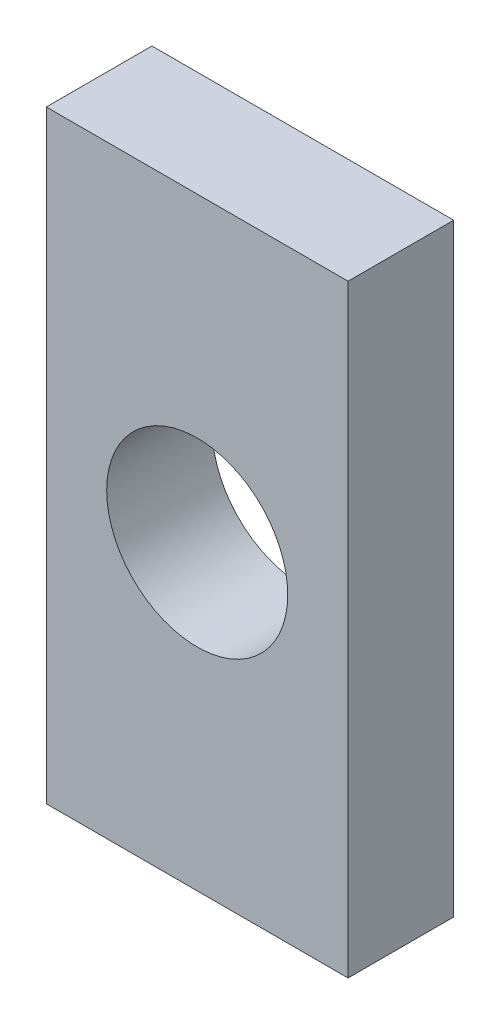
from build123d import *

# Parameters (mm, degrees)
SKETCH1_W           = 40
SKETCH1_H           = 80
SKETCH1_R           = 12
BOSS_EXTRUDE1_DEPTH = 14


with BuildPart() as part:
    # Sketch1 → Boss-Extrude1 (new body)
    with BuildSketch(Plane.XY):
        with Locations((20, 40)):
            Rectangle(SKETCH1_W, SKETCH1_H)
        with Locations((20, 40)):
            Circle(SKETCH1_R, mode=Mode.SUBTRACT)
    extrude(amount=BOSS_EXTRUDE1_DEPTH)


solid = part.part
